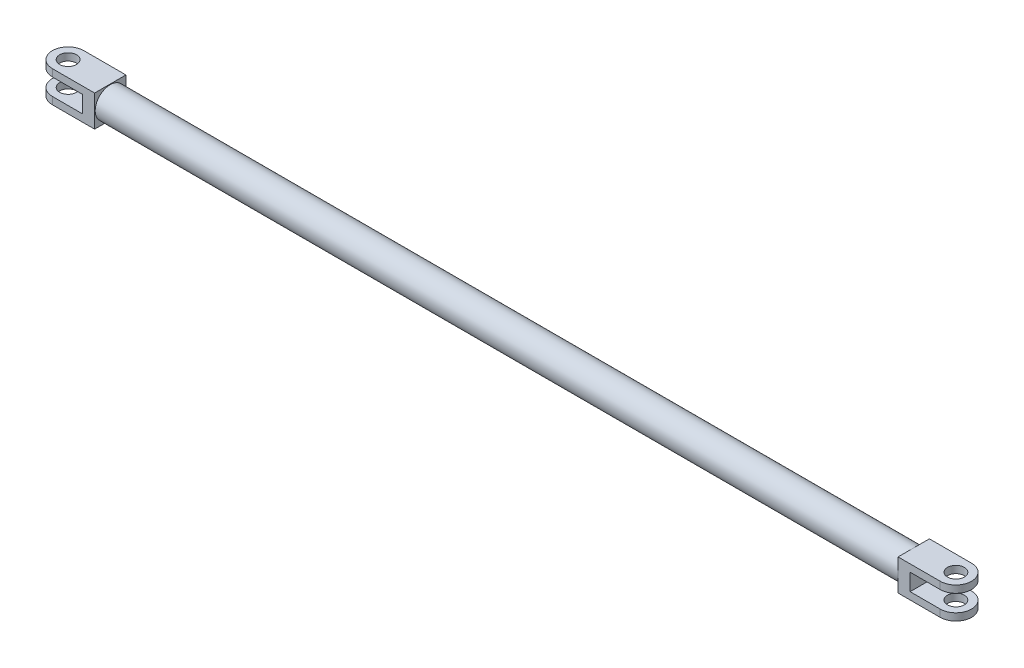
SolidWorks part; units mm, degrees
material "A3"
ref_plane "前视基准面" through (0, 0, 0) normal (0, 0, 1) x (1, 0, 0)
ref_plane "上视基准面" through (0, 0, 0) normal (0, 1, 0) x (1, 0, 0)
ref_plane "右视基准面" through (0, 0, 0) normal (1, 0, 0) x (0, 0, -1)
sketch "草图1" plane through (0, 0, 0) normal (0, 1, 0) x (1, 0, 0)
  line L0 (0, 13) -> (35, 13)
  line L1 (35, 13) -> (35, -13)
  line L2 (35, 0) -> (0, 0) construction
  line L3 (0, -13) -> (35, -13)
  circle A0 centre (0, 0) radius 7
  arc A1 (0, 13) -> (0, -13) centre (0, 0) ccw
  dimension "D1" = 14
  dimension "D2" = 26
  dimension "D3" = 35
extrude "凸台-拉伸1" add sketch "草图1" along normal mid plane 26
sketch "草图2" plane through (0, 0, 0) normal (0, 0, 1) x (1, 0, 0)
  line L1 (-25, -7) -> (25, -7)
  line L2 (-25, -7) -> (-25, 7)
  line L3 (-25, 7) -> (25, 7)
  line L4 (25, -7) -> (25, 7)
  line L5 (-25, -7) -> (25, 7) construction
  line L6 (-25, 7) -> (25, -7) construction
  point P0 (0, 0)
  dimension "D1" = 14
  dimension "D2" = 50
extrude "切除-拉伸1" cut sketch "草图2" against normal through all both and the other way through all
sketch "草图3" plane through (35, 0, 0) normal (1, 0, 0) x (0, 0, -1)
  circle A0 centre (0, 0) radius 9.5
  circle A1 centre (0, 0) radius 12.5
  dimension "D1" = 19
  dimension "D2" = 25
extrude "凸台-拉伸2" add sketch "草图3" along normal blind 667 separate body
ref_plane "基准面1" through (368.5, 0, 0) normal (1, 0, 0) x (0, 0, -1)
mirror "镜向1" about plane through (368.5, 0, 0) normal (1, 0, 0) of bodies 107
